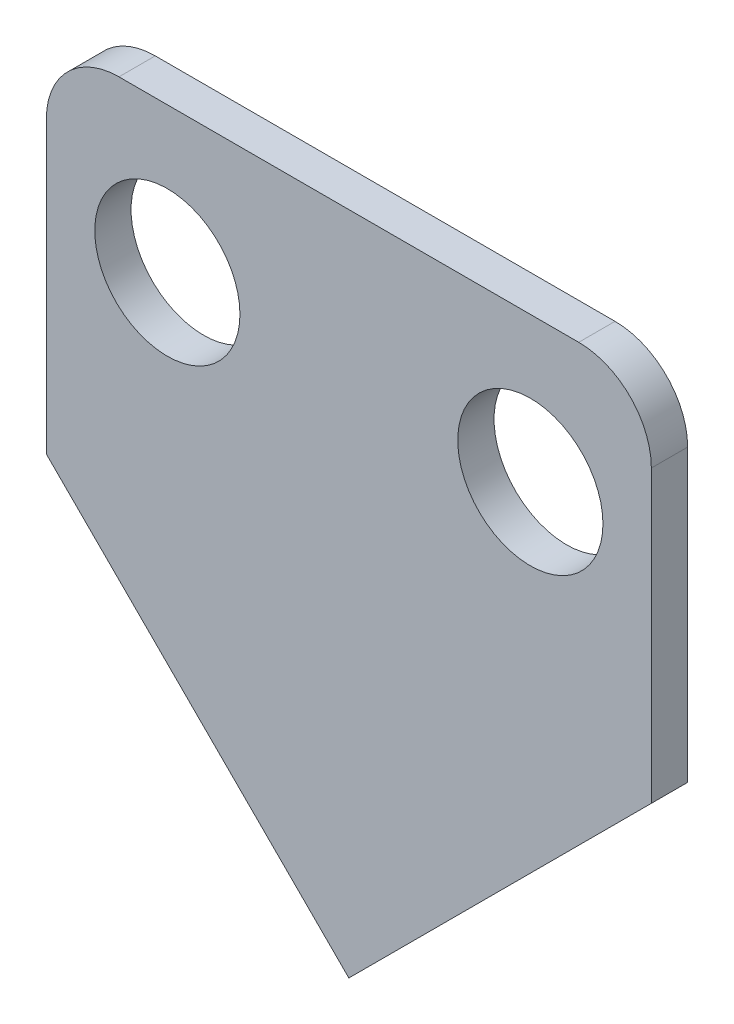
from build123d import *

# Parameters (mm, degrees)
EXTRUDE_1_DEPTH       = 1.5
HOLE_WIZARD_6_0_6_1_D = 6
FILLET_1_R            = 3


with BuildPart() as part:
    # 草图1 → 凸台-拉伸1 (new body)
    with BuildSketch(Plane.XY):
        Polygon((-12.5, 0), (12.5, 0), (12.5, -15), (0, -27.5), (-12.5, -15), align=None)
    extrude(amount=EXTRUDE_1_DEPTH)

    # Ø6.0 (6) 直径孔1 (through all)
    with Locations(Plane.XY.offset(1.5)):
        with Locations((-7.5, -6), (7.5, -6)):
            Hole(HOLE_WIZARD_6_0_6_1_D / 2)

    # 圆角1
    fillet_1_edges = [part.edges().sort_by_distance(p)[0] for p in [
        (-12.5, 0, 0.75),
        (12.5, 0, 0.75),
    ]]
    fillet(fillet_1_edges, radius=FILLET_1_R)


solid = part.part
